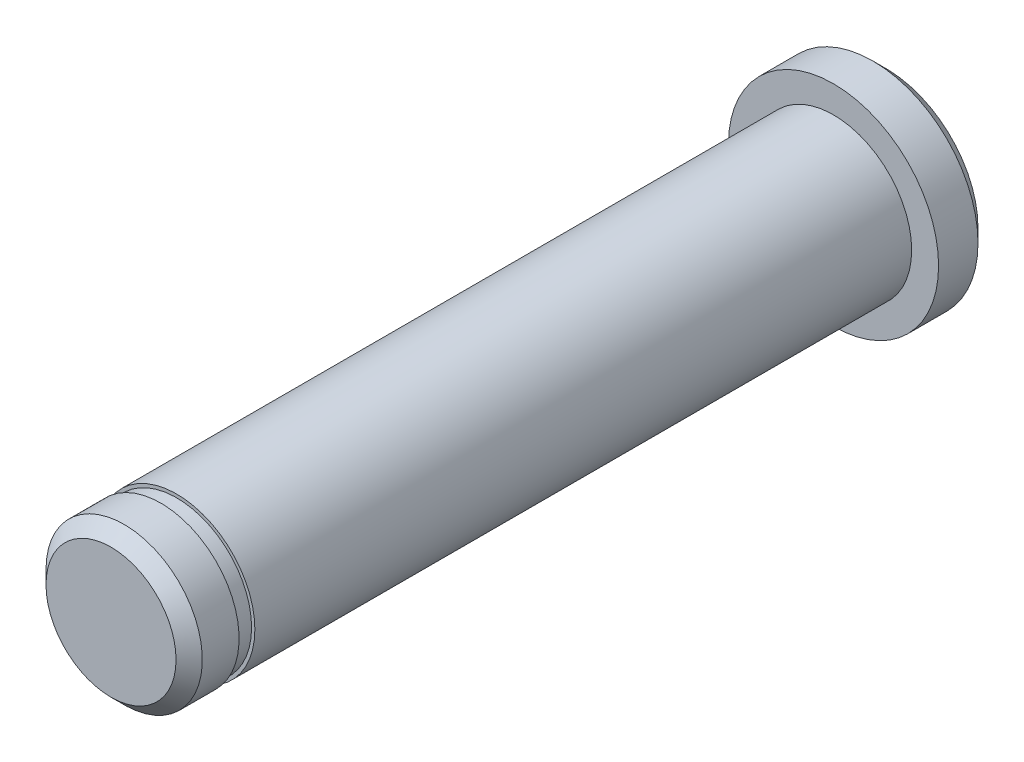
SolidWorks part; units mm, degrees
ref_plane "Front Plane" through (0, 0, 0) normal (0, 0, 1) x (1, 0, 0)
ref_plane "Top Plane" through (0, 0, 0) normal (0, 1, 0) x (1, 0, 0)
ref_plane "Right Plane" through (0, 0, 0) normal (1, 0, 0) x (0, 0, -1)
sketch "Sketch1" plane through (0, 0, 0) normal (0, 0, 1) x (1, 0, 0)
  circle A0 centre (0, 0) radius 4
  dimension "D1" = 8
extrude "Boss-Extrude1" add sketch "Sketch1" along normal blind 2
sketch "Sketch3" plane through (0, 0, 2) normal (0, 0, 1) x (1, 0, 0)
  circle A0 centre (0, 0) radius 2.975
  dimension "D1" = 5.95
extrude "Boss-Extrude2" add sketch "Sketch3" along normal blind 25
sketch "Sketch4" plane through (0, 0, 27) normal (0, 0, 1) x (1, 0, 0)
  circle A0 centre (0, 0) radius 2.85
  dimension "D1" = 5.7
extrude "Boss-Extrude3" add sketch "Sketch4" along normal blind 0.6
sketch "Sketch5" plane through (0, 0, 27.6) normal (0, 0, 1) x (1, 0, 0)
  circle A0 centre (0, 0) radius 2.975
  dimension "D1" = 5.95
extrude "Boss-Extrude4" add sketch "Sketch5" along normal blind 1.9
chamfer "Chamfer1" distance 0.5 angle 45 2 edges at (4, 0, 0) (2.975, 0, 29.5)
